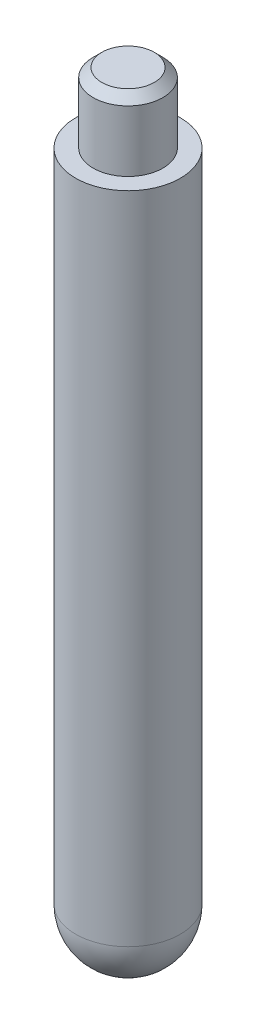
from build123d import *

# Parameters (mm, degrees)
CHAMFER1_SIZE = 1


with BuildPart() as part:
    # Sketch1 → Revolve1 (revolve)
    with BuildSketch(Plane.XY, mode=Mode.PRIVATE) as revolve1_sk:
        with BuildLine():
            Line((0, 90), (-4, 90))
            Line((-4, 90), (-4, 82))
            Line((-4, 82), (-6, 82))
            Line((-6, 82), (-6, 7))
            ThreePointArc((-6, 7), (-4.242640687, 2.757359313), (0, 1))
            Line((0, 1), (0, 90))
        make_face()
    revolve(revolve1_sk.sketch.rotate(Axis((0, 0, 0), (0, 1, 0)), 270), axis=Axis((0, 0, 0), (0, 1, 0)))

    # Chamfer1
    chamfer1_edges = [part.edges().sort_by_distance(p)[0] for p in [
        (0, 90, 4),
    ]]
    chamfer(chamfer1_edges, length=CHAMFER1_SIZE)


solid = part.part
